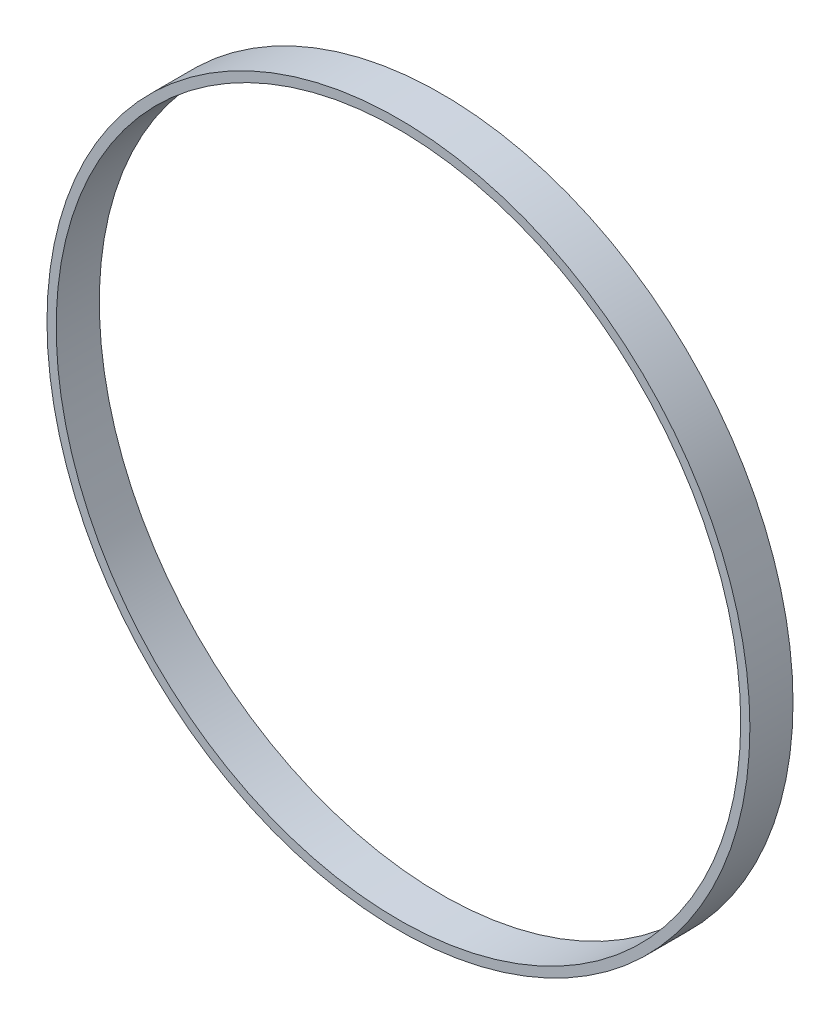
SolidWorks part; units mm, degrees
material "1023 碳钢板 (SS)"
ref_plane "前视基准面" through (0, 0, 0) normal (0, 0, 1) x (1, 0, 0)
ref_plane "上视基准面" through (0, 0, 0) normal (0, 1, 0) x (1, 0, 0)
ref_plane "右视基准面" through (0, 0, 0) normal (1, 0, 0) x (0, 0, -1)
sketch "草图1" plane through (0, 0, 0) normal (0, 0, 1) x (1, 0, 0)
  circle A0 centre (0, 0) radius 122.25
  circle A2 centre (0, 0) radius 119.05
  dimension "D1" = 244.5
  dimension "D2" = 238.1
extrude "凸台-拉伸1" add sketch "草图1" along normal blind 15 contours A0
